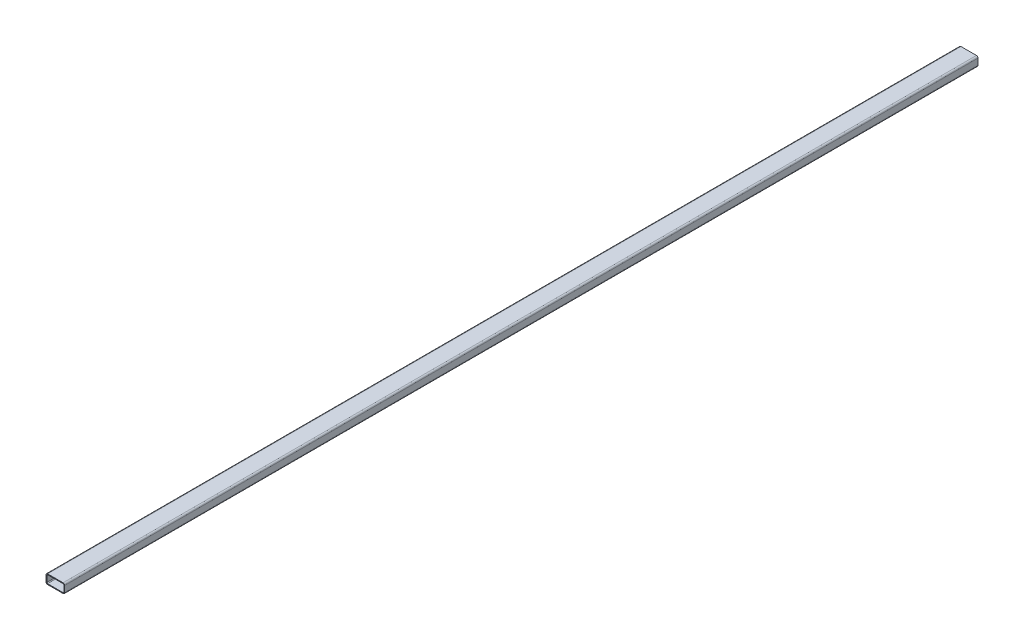
SolidWorks part; units mm, degrees
material "普通碳钢"
ref_plane "Front Plane" through (0, 0, 0) normal (0, 0, 1) x (1, 0, 0)
ref_plane "Top Plane" through (0, 0, 0) normal (0, 1, 0) x (1, 0, 0)
ref_plane "Right Plane" through (0, 0, 0) normal (1, 0, 0) x (0, 0, -1)
sketch "Sketch1" plane through (0, 0, 0) normal (0, 0, 1) x (1, 0, 0)
  line L0 (10, 55) -> (110, 55)
  line L1 (10, 0) -> (110, 0)
  line L2 (0, 10) -> (0, 50)
  line L3 (10, 60) -> (110, 60)
  line L4 (120, 10) -> (120, 50)
  line L5 (115, 10) -> (115, 50)
  line L6 (10, 5) -> (110, 5)
  line L7 (5, 10) -> (5, 50)
  arc A0 (120, 10) -> (110, 0) centre (110, 10) cw
  arc A1 (0, 50) -> (10, 60) centre (10, 50) cw
  arc A2 (120, 50) -> (110, 60) centre (110, 50) ccw
  arc A3 (10, 0) -> (0, 10) centre (10, 10) cw
  arc A4 (115, 50) -> (110, 55) centre (110, 50) ccw
  arc A5 (115, 10) -> (110, 5) centre (110, 10) cw
  arc A6 (10, 5) -> (5, 10) centre (10, 10) cw
  arc A7 (5, 50) -> (10, 55) centre (10, 50) cw
  point P7 (120, 0)
  point P10 (0, 60)
  point P13 (120, 60)
  point P16 (0, 0)
  dimension "D3" = 10
  dimension "D4" = 10
  dimension "D5" = 10
  dimension "D6" = 10
  dimension "D1" = 120
  dimension "D2" = 60
  dimension "D7" = 5
extrude "Boss-Extrude1" add sketch "Sketch1" along normal blind 5880
